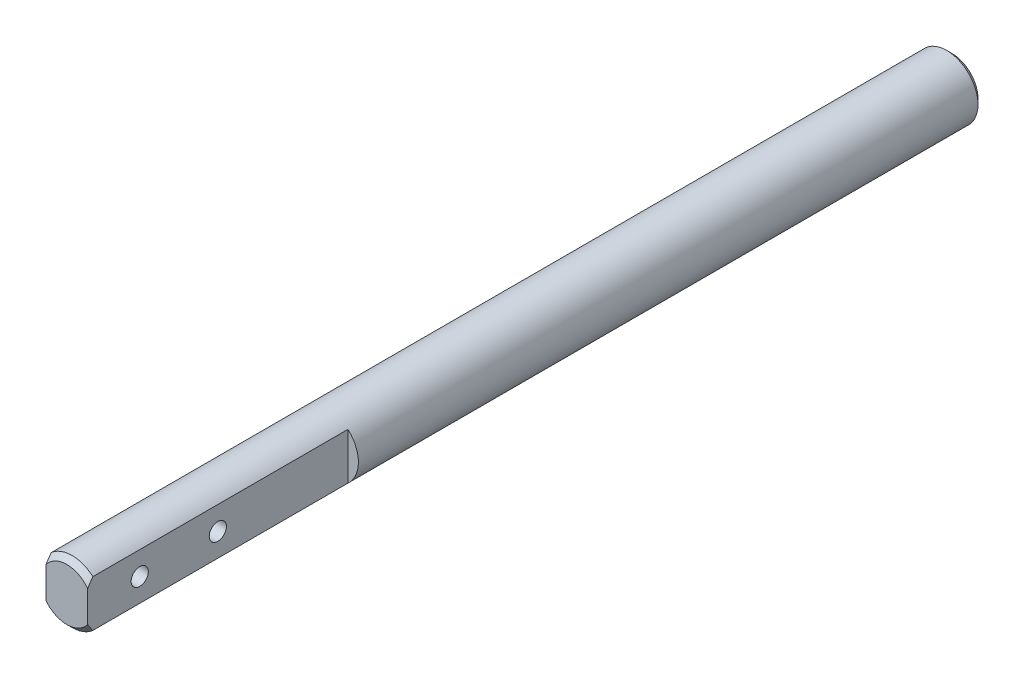
SolidWorks part; units mm, degrees
ref_plane "Front Plane" through (0, 0, 0) normal (0, 0, 1) x (1, 0, 0)
ref_plane "Top Plane" through (0, 0, 0) normal (0, 1, 0) x (1, 0, 0)
ref_plane "Right Plane" through (0, 0, 0) normal (1, 0, 0) x (0, 0, -1)
sketch "Sketch1" plane through (0, 0, 0) normal (0, 0, 1) x (1, 0, 0)
  circle A0 centre (0, 0) radius 6
extrude "Boss-Extrude1" add sketch "Sketch1" along normal blind 170
chamfer "Chamfer1" distance 1 angle 45 2 edges at (6, 0, 170) (6, 0, 0)
sketch "Sketch2" plane through (0, 0, 0) normal (0, 1, 0) x (1, 0, 0)
  line L0 (0, -174.8821) -> (0, -42.9077) construction
  line L1 (-6, -1) -> (-6, -169) construction
  line L2 (-6, -120) -> (-4, -120)
  line L3 (-6, -120) -> (-6, -170)
  line L4 (-6, -170) -> (-4, -170)
  line L5 (-4, -120) -> (-4, -170)
  line L6 (-5, -170) -> (5, -170) construction
  line L7 (4, -120) -> (4, -170)
  line L8 (6, -170) -> (4, -170)
  line L9 (6, -120) -> (6, -170)
  line L10 (6, -120) -> (4, -120)
  dimension "D1" = 2
  dimension "D2" = 50
extrude "Cut-Extrude1" cut sketch "Sketch2" against normal through all both and the other way through all
sketch "Sketch3" plane through (-4, 0, 0) normal (-1, 0, 0) x (0, 0, 1)
  line L0 (145, 0) -> (160, 0)
  line L1 (120, -4.4721) -> (120, 4.4721) construction
  dimension "D1" = 15
  dimension "D2" = 25
hole_wizard "M4 Tapped Hole1" positions "Sketch4" profile "Sketch5" tap size "M4" standard "GB" end condition through all
sketch "Sketch4" plane through (-4, 0, 0) normal (-1, 0, 0) x (0, 0, 1)
  point P0 (160, 0)
  point P3 (145, 0)
sketch "Sketch5" plane through (-4, 0, 160) normal (0, 1, 0) x (0, 0, 1)
  line L0 (0, 0) -> (0, 10)
  line L1 (0, 10) -> (1.65, 10)
  line L2 (1.65, 10) -> (1.65, 0.375)
  line L3 (1.65, 0.375) -> (2.025, 0)
  line L5 (2.025, 0) -> (0, 0)
  line L6 (-1.65, 0.375) -> (-2.025, 0) construction
  line L11 (0, -6.35) -> (0, 107.95) construction
  dimension "通孔螺纹孔钻头直径" = 3.3
  dimension "通孔螺纹孔钻头深度" = 10
  dimension "近端锥形沉头孔直径" = 4.05
  dimension "近端锥形沉头孔角度" = 90
cosmetic thread "Cosmetic thread 1" parameters "D2"=4
cosmetic thread "Cosmetic thread 2" parameters "D2"=4
